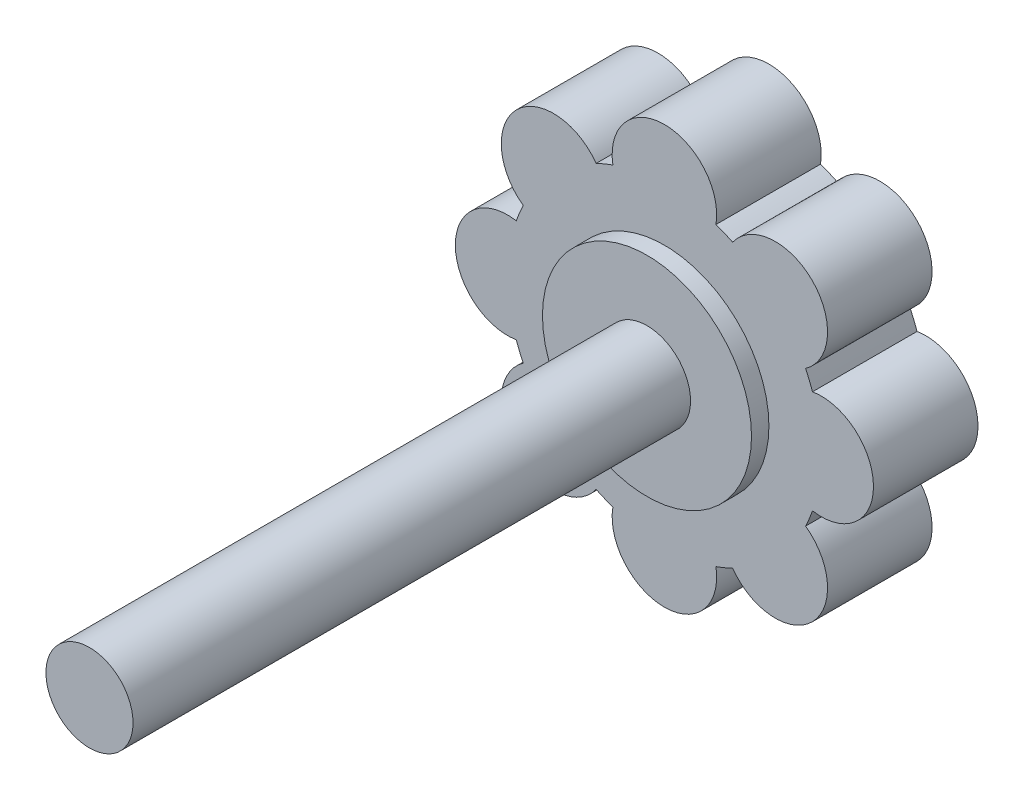
SolidWorks part; units mm, degrees
ref_plane "Front Plane" through (0, 0, 0) normal (0, 0, 1) x (1, 0, 0)
ref_plane "Top Plane" through (0, 0, 0) normal (0, 1, 0) x (1, 0, 0)
ref_plane "Right Plane" through (0, 0, 0) normal (1, 0, 0) x (0, 0, -1)
sketch "Sketch1" plane through (0, 0, 0) normal (0, 0, 1) x (1, 0, 0)
  arc A0 (-8.5, -2.958) -> (-8.1021, -3.9188) centre (0, 0) ccw
  arc A1 (2.958, 8.5) -> (-2.958, 8.5) centre (0, 9) ccw
  arc A2 (8.1021, 3.9188) -> (3.9188, 8.1021) centre (6.364, 6.364) ccw
  arc A3 (8.5, -2.958) -> (8.5, 2.958) centre (9, 0) ccw
  arc A4 (3.9188, -8.1021) -> (8.1021, -3.9188) centre (6.364, -6.364) ccw
  arc A5 (-2.958, -8.5) -> (2.958, -8.5) centre (0, -9) ccw
  arc A6 (-8.1021, -3.9188) -> (-3.9188, -8.1021) centre (-6.364, -6.364) ccw
  arc A7 (-8.5, 2.958) -> (-8.5, -2.958) centre (-9, 0) ccw
  arc A8 (-3.9188, 8.1021) -> (-8.1021, 3.9188) centre (-6.364, 6.364) ccw
  arc A9 (-8.1021, 3.9188) -> (-8.5, 2.958) centre (0, 0) ccw
  arc A10 (-2.958, 8.5) -> (-3.9188, 8.1021) centre (0, 0) ccw
  arc A11 (3.9188, 8.1021) -> (2.958, 8.5) centre (0, 0) ccw
  arc A12 (8.5, 2.958) -> (8.1021, 3.9188) centre (0, 0) ccw
  arc A13 (8.1021, -3.9188) -> (8.5, -2.958) centre (0, 0) ccw
  arc A14 (2.958, -8.5) -> (3.9188, -8.1021) centre (0, 0) ccw
  arc A15 (-3.9188, -8.1021) -> (-2.958, -8.5) centre (0, 0) ccw
  point P22 (0, 0)
  dimension "D1" = 18
  dimension "D2" = 6
  dimension "D3" = 8
extrude "Boss-Extrude1" add sketch "Sketch1" along normal blind 6
sketch "Sketch2" plane through (0, 0, 6) normal (0, 0, 1) x (1, 0, 0)
  circle A0 centre (0, 0) radius 2.5
  dimension "D1" = 5
extrude "Boss-Extrude2" add sketch "Sketch2" along normal blind 33
sketch "Sketch3" plane through (0, 0, 6) normal (0, 0, 1) x (1, 0, 0)
  circle A0 centre (0, 0) radius 6
  dimension "D1" = 12
extrude "Boss-Extrude3" add sketch "Sketch3" along normal mid plane 2
sketch "Sketch4" plane through (0, 0, 0) normal (0, 0, -1) x (-1, 0, 0)
  circle A0 centre (0, 0) radius 3.7046
extrude "Cut-Extrude1" cut sketch "Sketch4" against normal blind 0.2
